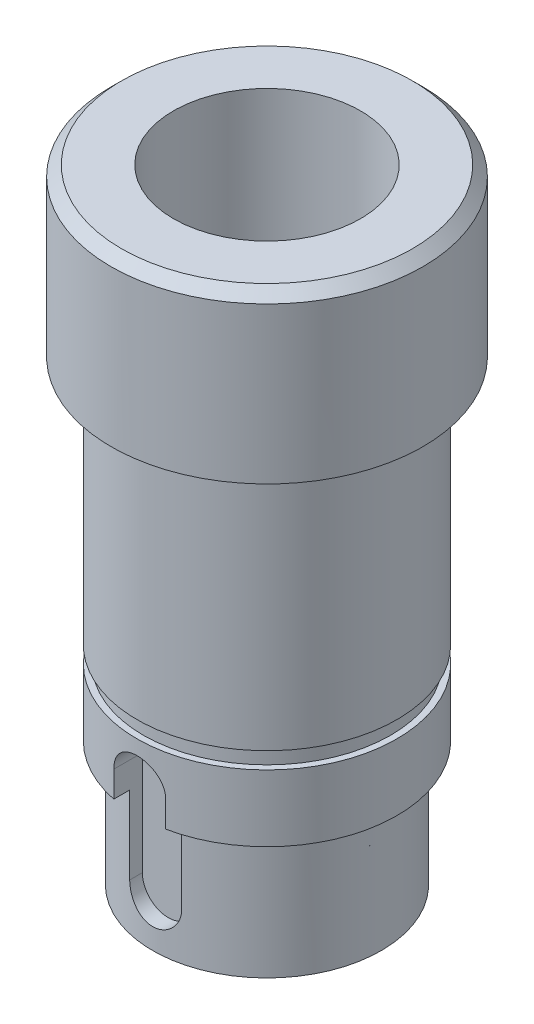
from build123d import *

# Parameters (mm, degrees)
SKETCH2_W          = 4.874466188
SKETCH2_H          = 1.6
SKETCH3_R          = 9
CUT_EXTRUDE1_DEPTH = 20
M16_TAPPED_HOLE2_D = 14
CHAMFER1_SIZE      = 1
CUT_EXTRUDE2_START = 12.5
CUT_EXTRUDE2_DEPTH = 3
SKETCH10_R         = 15
SKETCH10_R_2       = 11
CUT_EXTRUDE3_DEPTH = 12


with BuildPart() as part:
    # Sketch1 → Revolve1 (revolve)
    with BuildSketch(Plane.XY, mode=Mode.PRIVATE) as revolve1_sk:
        Polygon((6, 60), (15, 60), (15, 44), (12.5, 44), (12.5, 0), (6, 0), align=None)
    revolve(revolve1_sk.sketch.rotate(Axis((0, 0, 0), (0, 1, 0)), 90), axis=Axis((0, 0, 0), (0, 1, 0)))

    # Sketch2 → Cut-Revolve1 (revolve, cut)
    with BuildSketch(Plane.XY, mode=Mode.PRIVATE) as cut_revolve1_sk:
        with Locations((-14.337233094, 19.2)):
            Rectangle(SKETCH2_W, SKETCH2_H)
    revolve(cut_revolve1_sk.sketch.rotate(Axis((0, 0, 0), (0, 1, 0)), 270), axis=Axis((0, 0, 0), (0, 1, 0)), mode=Mode.SUBTRACT)

    # Sketch3 → Cut-Extrude1 (cut)
    with BuildSketch(Plane(origin=(0, 60, 0), x_dir=(1, 0, 0), z_dir=(0, 1, 0))):
        with Locations(Location((0, 0, 0), (0, 0, 270))):
            Circle(SKETCH3_R)
    extrude(amount=-CUT_EXTRUDE1_DEPTH, mode=Mode.SUBTRACT)

    # M16 Tapped Hole2 (through all)
    with Locations(Plane(origin=(0, 0, 0), x_dir=(-1, 0, 0), z_dir=(0, -1, 0))):
        with Locations((0, 0)):
            Hole(M16_TAPPED_HOLE2_D / 2)

    # Chamfer1
    chamfer1_edges = [part.edges().sort_by_distance(p)[0] for p in [
        (0, 0, 12.5),
        (0, 60, 15),
    ]]
    chamfer(chamfer1_edges, length=CHAMFER1_SIZE)

    # Sketch8 → Cut-Extrude2 (cut)
    with BuildSketch(Plane.XY.offset(CUT_EXTRUDE2_START)):
        with BuildLine():
            Line((2.5, 14.5), (2.5, 4.5))
            ThreePointArc((2.5, 4.5), (0, 2), (-2.5, 4.5))
            Line((-2.5, 4.5), (-2.5, 14.5))
            ThreePointArc((-2.5, 14.5), (0, 17), (2.5, 14.5))
        make_face()
    extrude(amount=-CUT_EXTRUDE2_DEPTH, mode=Mode.SUBTRACT)

    # Sketch10 → Cut-Extrude3 (cut)
    with BuildSketch(Plane.XZ):
        with Locations(Location((0, 0, 0), (0, 0, 270))):
            Circle(SKETCH10_R)
        with Locations(Location((0, 0, 0), (0, 0, 270))):
            Circle(SKETCH10_R_2, mode=Mode.SUBTRACT)
    extrude(amount=-CUT_EXTRUDE3_DEPTH, mode=Mode.SUBTRACT)


solid = part.part
